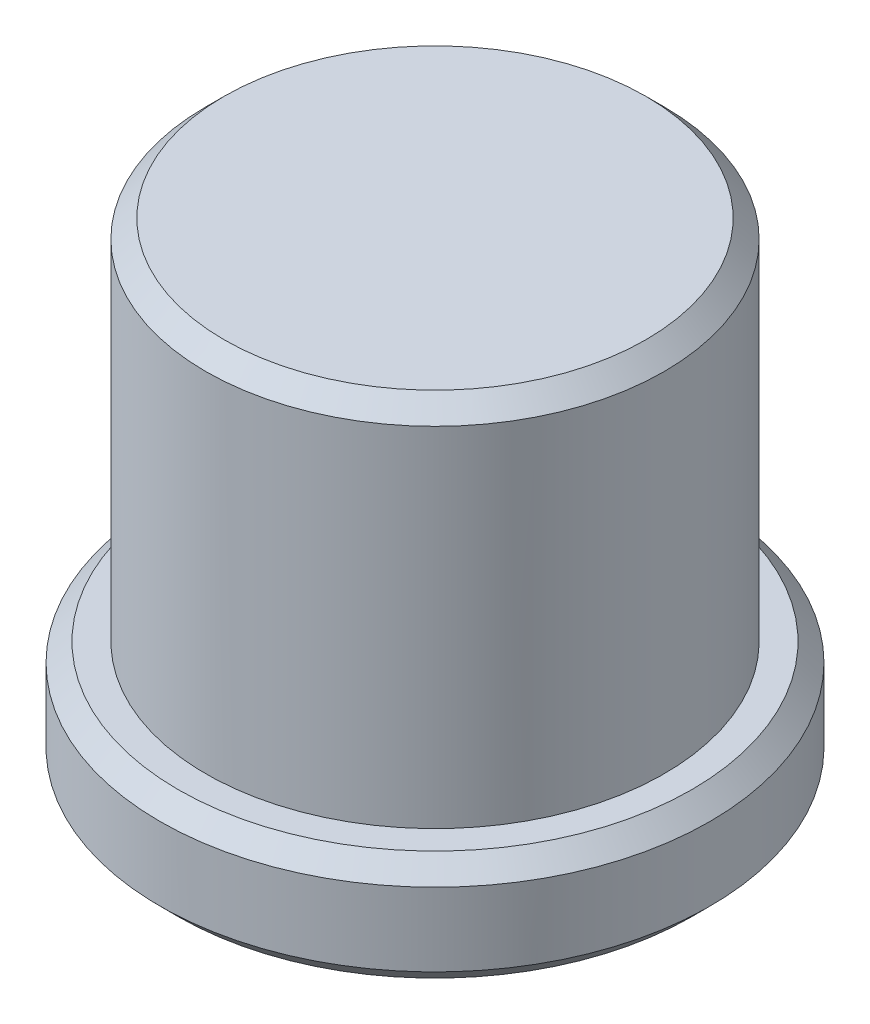
from build123d import *

# Parameters (mm, degrees)
CHAMFER1_SIZE = 0.5


with BuildPart() as part:
    # Sketch1 → Revolve1 (revolve)
    with BuildSketch(Plane(origin=(0, 0, 0), x_dir=(0, 0, -1), z_dir=(1, 0, 0))):
        Polygon((0, 13), (6.25, 13), (6.25, 3), (7.5, 3), (7.5, 0), (0, 0), align=None)
    revolve(axis=Axis((0, 0, 0), (0, 1, 0)))

    # Chamfer1
    chamfer1_edges = [part.edges().sort_by_distance(p)[0] for p in [
        (0, 0, 7.5),
        (0, 3, 7.5),
        (0, 13, 6.25),
    ]]
    chamfer(chamfer1_edges, length=CHAMFER1_SIZE)


solid = part.part
